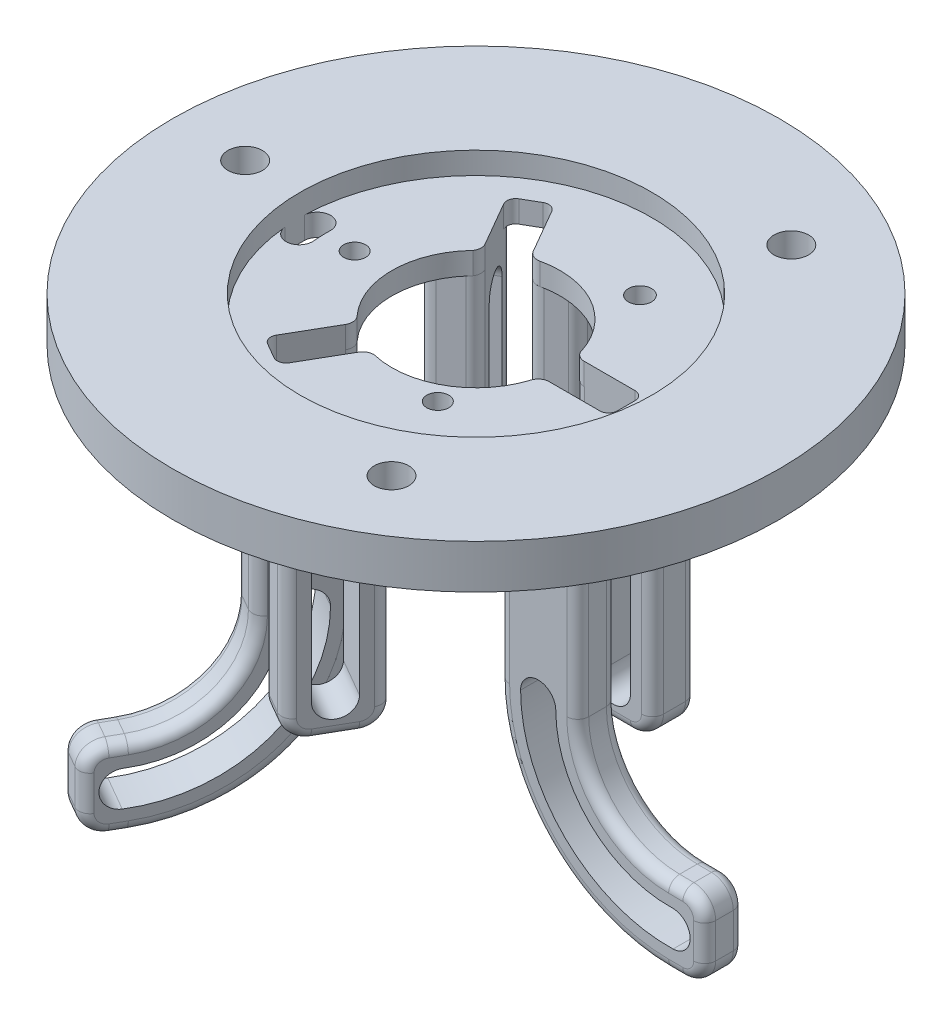
SolidWorks part; units mm, degrees
ref_plane "Front Plane" through (0, 0, 0) normal (0, 0, 1) x (1, 0, 0)
ref_plane "Top Plane" through (0, 0, 0) normal (0, 1, 0) x (1, 0, 0)
ref_plane "Right Plane" through (0, 0, 0) normal (1, 0, 0) x (0, 0, -1)
sketch "Sketch1" plane through (0, 0, 0) normal (0, 1, 0) x (1, 0, 0)
  circle A0 centre (0, 0) radius 138
extrude "Boss-Extrude1" add sketch "Sketch1" along normal blind 20
sketch "Sketch2" plane through (0, 0, 0) normal (0, 0, 1) x (1, 0, 0)
  line L0 (-138, 0) -> (138, 0) construction
  line L1 (62.2913, -161.1366) -> (62.2913, -17.2466)
  line L2 (54.2913, -100) -> (148.881, -100) construction
  line L3 (54.2913, -161.1366) -> (148.881, -161.1366) construction
  line L4 (113.6373, -189.6328) -> (113.6373, -71.1378) construction
  line L5 (113.6373, -71.1378) -> (113.6373, 30.2376) construction
  line L6 (138, 20) -> (138, 0) construction
  line L7 (54.2913, -161.1366) -> (54.2913, -17.2466) construction
  line L8 (46.2913, -161.1366) -> (46.2913, -17.2466)
  line L9 (36.2913, 0) -> (36.2913, -145.1821)
  line L10 (36.2913, -145.1821) -> (89.2746, -189.6328)
  line L11 (89.2746, -189.6328) -> (138, -189.6328)
  line L12 (82.2913, 0) -> (82.2913, -93.731)
  line L13 (82.2913, -93.731) -> (138, -149.4397)
  line L14 (138, -149.4397) -> (138, -189.6328)
  line L15 (138, 0) -> (138, -271.006) construction
  line L16 (36.2913, 0) -> (82.2913, 0)
  arc A0 (54.2913, -100) -> (113.6373, -159.346) centre (113.6373, -100) ccw construction
  arc A1 (54.2913, -161.1366) -> (113.6373, -220.4826) centre (113.6373, -161.1366) ccw construction
  arc A2 (62.2913, -161.1366) -> (113.6373, -212.4826) centre (113.6373, -161.1366) ccw
  arc A3 (46.2913, -100) -> (113.6373, -167.346) centre (113.6373, -100) ccw
  arc A4 (46.2913, -161.1366) -> (113.6373, -228.4826) centre (113.6373, -161.1366) ccw
  arc A5 (62.2913, -100) -> (113.6373, -151.346) centre (113.6373, -100) ccw
  arc A6 (113.6373, -212.4826) -> (113.6373, -228.4826) centre (113.6373, -220.4826) cw
  arc A7 (62.2913, -17.2466) -> (46.2913, -17.2466) centre (54.2913, -17.2466) ccw
  arc A8 (46.2913, -100) -> (62.2913, -100) centre (54.2913, -100) cw
  arc A9 (113.6373, -167.346) -> (113.6373, -151.346) centre (113.6373, -159.346) ccw
  circle A10 centre (54.2913, -161.1366) radius 8
  point P12 (113.6373, -100)
  point P14 (113.6373, -161.1366)
  point P15 (113.6373, -161.1366)
  dimension "D6" = 10
  dimension "D1" = 100
  dimension "D2" = 24.3627
  dimension "D3" = 61.1366
  dimension "D7" = 20
  dimension "D8" = 135
  dimension "D4" = 8
  dimension "D5" = 8
extrude "Boss-Extrude2" add sketch "Sketch2" along normal blind 10 and the other way blind 8 from offset 16 contours L16 L12 L13 L14 L11 L10 L9
sketch "Sketch3" plane through (0, 0, 26) normal (0, 0, 1) x (1, 0, 0)
  line L0 (54.2913, -17.2466) -> (54.2913, -110.5186) construction
  line L1 (46.2913, -17.2466) -> (46.2913, -110.5186)
  line L2 (62.2913, -17.2466) -> (62.2913, -110.5186)
  arc A0 (46.2913, -17.2466) -> (62.2913, -17.2466) centre (54.2913, -17.2466) cw
  arc A1 (46.2913, -110.5186) -> (62.2913, -110.5186) centre (54.2913, -110.5186) ccw
  dimension "D1" = 8
  dimension "D2" = 8
sketch "Sketch4" plane through (0, 0, 8) normal (0, 0, 1) x (1, 0, 0)
  arc A0 (54.2913, -100) -> (115.4184, -159.3192) centre (113.6373, -100) ccw
  arc A1 (54.2913, -100) -> (113.6373, -159.346) centre (113.6373, -100) ccw construction
  arc A2 (54.2913, -161.1366) -> (115.3389, -220.4582) centre (113.6373, -161.1366) ccw
  arc A3 (54.2913, -161.1366) -> (113.6373, -220.4826) centre (113.6373, -161.1366) ccw construction
  arc A4 (46.2913, -161.1366) -> (115.5682, -228.4549) centre (113.6373, -161.1366) ccw
  arc A5 (46.2913, -100) -> (115.6585, -167.3156) centre (113.6373, -100) ccw
  arc A6 (62.2913, -161.1366) -> (115.1095, -212.4615) centre (113.6373, -161.1366) ccw
  arc A7 (62.2913, -100) -> (115.1783, -151.3229) centre (113.6373, -100) ccw
  arc A8 (46.2913, -161.1366) -> (62.2913, -161.1366) centre (54.2913, -161.1366) cw
  arc A9 (115.5682, -228.4549) -> (115.1095, -212.4615) centre (115.3389, -220.4582) ccw
  arc A10 (46.2913, -100) -> (62.2913, -100) centre (54.2913, -100) cw
  arc A11 (115.6585, -167.3156) -> (115.1783, -151.3229) centre (115.4184, -159.3192) ccw
  dimension "D1" = 8
  dimension "D2" = 8
extrude "Cut-Extrude5" cut sketch "Sketch4" along normal blind 34
ref_plane "Plane1" through (0, 0, 42) normal (0, 0, 1) x (1, 0, 0)
sketch "Sketch7" plane through (0, 0, 42) normal (0, 0, 1) x (1, 0, 0)
  line L0 (36.2913, 0) -> (36.2913, -125.9674)
  line L1 (36.2913, 0) -> (36.2913, -145.1821) construction
  line L2 (36.2913, -125.9674) -> (82.2913, -125.9674)
  line L3 (82.2913, -125.9674) -> (82.2913, 0)
  line L4 (82.2913, 0) -> (36.2913, 0)
extrude "Boss-Extrude3" add sketch "Sketch7" along normal blind 20 from offset 70 contours L0 L2 L3 L4 offset against normal yes
extrude "Cut-Extrude6" cut sketch "Sketch3" along normal blind 45 from offset 72 offset against normal yes
sketch "Sketch8" plane through (0, 0, 26) normal (0, 0, 1) x (1, 0, 0)
  line L0 (130.0411, -141.4808) -> (130.0411, -169.783)
  line L1 (82.2913, -93.731) -> (138, -149.4397) construction
  line L2 (130.0411, -169.783) -> (130.0618, -195.2719)
  line L10 (130.065, -199.2899) -> (144.6927, -199.2899)
  line L11 (144.6927, -199.2899) -> (138, -149.4397)
  line L12 (138, -149.4397) -> (130.0411, -141.4808)
  line L13 (130.0618, -195.2719) -> (144.6927, -199.2899)
  line M11 (89.2746, -189.6328) -> (138, -189.6328)
  line M12 (138, -189.6328) -> (138, -149.4397)
  line M13 (138, -149.4397) -> (82.2913, -93.731)
extrude "Cut-Extrude7" cut sketch "Sketch8" against normal blind 72 contours L0 L2 M11 M12 M13
pattern_circular "CirPattern1" count 3 over 360 about axis through (0, 0, 0) along (0, 1, 0) of "Boss-Extrude3", "Cut-Extrude6", "Cut-Extrude5", "Boss-Extrude2", "Cut-Extrude7"
sketch "Sketch9" plane through (0, 0, -28) normal (0, 0, -1) x (-1, 0, 0)
  line L4 (-72.2913, -43.2737) -> (-72.2913, 0)
  line L5 (-82.2913, 0) -> (-36.2913, 0) construction
  line L6 (-72.2913, -43.2737) -> (-72.2913, -125.9674)
  line L7 (-36.2913, -125.9674) -> (-82.2913, -125.9674) construction
  line L8 (-72.2913, -125.9674) -> (-82.2913, -125.9674)
  line L9 (-82.2913, -125.9674) -> (-82.2913, 0)
  line L10 (-82.2913, 0) -> (-72.2913, 0)
extrude "Cut-Extrude8" cut sketch "Sketch9" against normal blind 27
sketch "Sketch11" plane through (0, 0, 26) normal (0, 0, 1) x (1, 0, 0)
  line L0 (36.2913, -100) -> (36.2913, -145.1821)
  line L1 (36.2913, -145.1821) -> (89.2746, -189.6328)
  line L2 (89.2746, -189.6328) -> (130.0572, -189.6328)
  line L3 (130.0572, -189.6328) -> (134.4943, -177.346)
  line L5 (72.2873, -100) -> (72.2873, 0)
  line L6 (36.2913, 0) -> (82.2913, 0) construction
  line L7 (72.2873, 0) -> (138, 0)
  line L8 (138, 0) -> (154.9873, -100)
  line L9 (113.6373, -141.35) -> (130.0411, -141.4808)
  line L10 (130.0411, -141.4808) -> (142.1558, -129.9419)
  line L11 (113.6373, -177.346) -> (134.4943, -177.346)
  arc A0 (36.2913, -100) -> (113.6373, -177.346) centre (113.6373, -100) ccw
  arc A1 (72.2873, -100) -> (113.6373, -141.35) centre (113.6373, -100) ccw
  arc A2 (142.1558, -129.9419) -> (154.9873, -100) centre (113.6373, -100) ccw
  dimension "D1" = 82.7
extrude "Cut-Extrude10" cut sketch "Sketch11" against normal blind 27
pattern_circular "CirPattern4" count 3 over 360 about axis through (0, 20, 0) along (0, -1, 0) of "Cut-Extrude8"
pattern_circular "CirPattern5" count 3 over 360 about axis through (0, 0, 0) along (0, 1, 0) of "Cut-Extrude10"
fillet "Fillet2" radius 10 21 edges at (-2.5572, -125.9674, 40.4292) (-33.7341, -125.9674, -22.4292) (-79.743, -169.783, 104.1189) (-79.743, -141.4808, 104.1189) (-71.9503, -173.5645, 108.6215) (-87.5387, -173.5645, 99.6215) (-50.2981, -169.783, -121.1189) (-50.2981, -141.4808, -121.1189) (-58.0939, -173.5645, -116.6215) (-42.5054, -173.5645, -125.6215) (72.2913, -125.9674, -18) (130.0472, -177.346, 17) (-51.7341, -125.9674, -53.6061) (-20.5572, -125.9674, 71.6061) (-79.746, -177.346, 104.1242) (-50.3012, -177.346, -121.1242) (36.2913, -125.9674, -18) (130.0411, -169.783, 17) (130.0411, -141.4808, 17) (130.0441, -173.5645, 8) (130.0441, -173.5645, 26)
sketch "Sketch12" plane through (0, 20, 0) normal (0, 1, 0) x (1, 0, 0)
  line L0 (0, 0) -> (-105, 0) construction
  line L1 (0, 0) -> (0, 105) construction
  circle A0 centre (0, 0) radius 105 construction
  circle A2 centre (-105, 0) radius 7.875
  dimension "D1" = 210
  dimension "D2" = 15.75
  dimension "D3" = 90
extrude "Cut-Extrude11" cut sketch "Sketch12" against normal blind 27
pattern_circular "CirPattern8" count 3 over 360 about axis through (0, 0, 0) along (0, 1, 0) of "Cut-Extrude11"
fillet "Fillet3" radius 5 84 edges at (-25.0739, -50, 27.4292) (36.2913, -50, 26) (-40.6623, -50, 18.4292) (-11.2175, -50, -35.4292) (4.371, -50, -44.4292) (6.103, -57.9837, 45.4292) (-11.2175, -57.9837, 35.4292) (-42.3944, -57.9837, -17.4292) (-25.0739, -57.9837, -27.4292) (72.2913, -57.9837, -8) (58.9454, -154.6919, 8) (58.9454, -154.6919, 26) (72.2873, -50, 26) (84.3984, -129.2389, 26) (116.879, -141.3758, 26) (84.3984, -129.2389, 8) (72.2873, -50, 8) (116.879, -141.3758, 8) (-43.0739, -57.9837, -58.6061) (-29.2175, -57.9837, 66.6061) (-22.5445, -154.6919, -55.0482) (-6.9561, -154.6919, -64.0482) (-58.6603, -50, 49.6026) (-64.7159, -129.2389, 60.0912) (-80.9562, -141.3758, 88.2202) (-49.1274, -129.2389, 69.0912) (-43.0719, -50, 58.6026) (-65.3677, -141.3758, 97.2202) (-36.4009, -154.6919, 47.0482) (-51.9894, -154.6919, 38.0482) (36.2913, -57.9837, -28) (-13.627, -50, -75.6026) (-19.6826, -129.2389, -86.0912) (-35.9229, -141.3758, -114.2202) (-35.271, -129.2389, -77.0912) (-29.2155, -50, -66.6026) (-51.5113, -141.3758, -105.2202) (36.2913, -57.9837, -8) (-42.5039, -159.3737, -125.6189) (-58.0923, -159.3737, -116.6189) (-35.9029, -177.346, -114.1857) (-41.0394, -174.4171, -123.0823) (-41.0535, -144.3585, -123.1067) (-51.4914, -177.346, -105.1857) (-56.6279, -174.4171, -114.0823) (-56.6419, -144.3585, -114.1067) (-87.5372, -159.3737, 99.6189) (-71.9487, -159.3737, 108.6189) (-80.9363, -177.346, 88.1857) (-86.0727, -174.4171, 97.0823) (-86.0868, -144.3585, 97.1067) (-65.3478, -177.346, 97.1857) (-70.4843, -174.4171, 106.0823) (-70.4983, -144.3585, 106.1067) (-60.3944, -57.9837, -48.6061) (-51.3944, -125.9674, -33.0177) (-43.8588, -123.0385, -19.9657) (-58.9299, -123.0385, -46.0696) (-34.0739, -125.9674, -43.0177) (-26.5383, -123.0385, -29.9657) (-41.6094, -123.0385, -56.0696) (-2.897, -125.9674, 61.0177) (-20.2175, -125.9674, 51.0177) (-11.897, -57.9837, 76.6061) (-10.4325, -123.0385, 74.0696) (4.6386, -123.0385, 47.9657) (-27.753, -123.0385, 64.0696) (-12.6819, -123.0385, 37.9657) (54.2913, -125.9674, -28) (54.2913, -125.9674, -8) (72.2913, -57.9837, -28) (69.3624, -123.0385, -28) (39.2203, -123.0385, -28) (69.3624, -123.0385, -8) (39.2203, -123.0385, -8) (130.0411, -159.3737, 26) (130.0411, -159.3737, 8) (116.8392, -177.346, 26) (127.1121, -174.4171, 26) (127.1403, -144.3585, 26) (116.8392, -177.346, 8) (127.1121, -174.4171, 8) (127.1403, -144.3585, 8) (36.2913, -50, 8)
sketch "Sketch13" plane through (0, 0, 0) normal (0, -1, 0) x (1, 0, 0)
  line L0 (-39.0867, 51.7001) -> (-25.6504, 28.4278)
  line L2 (-27.5739, 31.7593) -> (-40.5719, 54.2725) construction
  line L4 (-25.2303, 59.7001) -> (-11.794, 36.4278)
  line L6 (-37.6226, 57.1642) -> (-30.6944, 61.1642)
  line L7 (64.3169, -8) -> (37.4444, -8)
  line L8 (68.3169, 4) -> (68.3169, -4)
  line L9 (64.3169, 8) -> (37.4444, 8)
  line L10 (-39.0867, -51.7001) -> (-25.6504, -28.4278)
  line L11 (-30.6944, -61.1642) -> (-37.6226, -57.1642)
  line L12 (-25.2303, -59.7001) -> (-11.794, -36.4278)
  arc A0 (-25.6504, 28.4278) -> (-25.6504, -28.4278) centre (0, 0) ccw
  arc A1 (37.4444, 8) -> (-11.794, 36.4278) centre (0, 0) ccw
  arc A2 (-11.794, -36.4278) -> (37.4444, -8) centre (0, 0) ccw
  arc A3 (-25.2303, 59.7001) -> (-30.6944, 61.1642) centre (-28.6944, 57.7001) ccw
  arc A4 (68.3169, 4) -> (64.3169, 8) centre (64.3169, 4) ccw
  arc A5 (68.3169, -4) -> (64.3169, -8) centre (64.3169, -4) cw
  arc A6 (-37.6226, -57.1642) -> (-39.0867, -51.7001) centre (-35.6226, -53.7001) cw
  arc A7 (-39.0867, 51.7001) -> (-37.6226, 57.1642) centre (-35.6226, 53.7001) cw
  arc A8 (-30.6944, -61.1642) -> (-25.2303, -59.7001) centre (-28.6944, -57.7001) ccw
  point P18 (0, 0)
  dimension "D2" = 4
  dimension "D3" = 4
  dimension "D4" = 4
  dimension "D1" = 3
extrude "Cut-Extrude12" cut sketch "Sketch13" against normal blind 27
sketch "Sketch14" plane through (0, 0, 0) normal (0, -1, 0) x (1, 0, 0)
  line L0 (-27.5739, 31.7593) -> (-13.7175, 39.7593)
  line L3 (41.2913, 8) -> (41.2913, -8)
  line L4 (-13.7175, -39.7593) -> (-27.5739, -31.7593)
  arc A0 (-13.7175, 39.7593) -> (-8.9941, 37.2181) centre (-9.3271, 42.2593) ccw
  arc A1 (-27.5739, 31.7593) -> (-28.1914, 25.9099) centre (-31.9042, 29.2592) cw
  arc A2 (-28.219, 25.8798) -> (-28.219, -25.8798) centre (0, 0) ccw construction
  arc A3 (-25.6504, 28.4278) -> (-28.219, 25.8798) centre (0, 0) ccw construction
  arc A4 (-28.1914, 25.9099) -> (-27.7347, -26.3982) centre (0, 0) ccw
  arc A6 (41.2913, 8) -> (36.5344, 11.4595) centre (41.2913, 13.0003) cw
  arc A7 (41.2913, -8) -> (36.7289, -10.8199) centre (41.2612, -13.0522) ccw
  arc A8 (-13.7175, -39.7593) -> (-8.343, -37.3694) centre (-9.3871, -42.2595) cw
  arc A9 (-27.5739, -31.7593) -> (-27.7347, -26.3982) centre (-31.9341, -29.2072) ccw
  arc A10 (36.5344, 11.4595) -> (-8.9941, 37.2181) centre (0, 0) ccw
  arc A11 (-8.343, -37.3694) -> (36.7289, -10.8199) centre (0, 0) ccw
  point P31 (0, 0)
  dimension "D1" = 3
extrude "Cut-Extrude13" cut sketch "Sketch14" against normal blind 27
sketch "Sketch17" plane through (0, 20, 0) normal (0, 1, 0) x (1, 0, 0)
  circle A0 centre (0, 0) radius 80
  dimension "D1" = 160
extrude "Cut-Extrude14" cut sketch "Sketch17" against normal blind 10
sketch "Sketch18" plane through (0, 10, 0) normal (0, 1, 0) x (1, 0, 0)
  arc A0 (-73.6973, -6.6862) -> (-73.9778, 1.812) centre (0, 0) cw construction
  arc A1 (-79.976, 1.959) -> (-79.6728, -7.2283) centre (0, 0) ccw
  arc A2 (-67.9796, 1.6651) -> (-67.7219, -6.144) centre (0, 0) ccw
  arc A3 (-67.9796, 1.6651) -> (-79.976, 1.959) centre (-73.9778, 1.812) ccw
  arc A4 (-79.6728, -7.2283) -> (-67.7219, -6.144) centre (-73.6973, -6.6862) ccw
  circle A5 centre (0, 0) radius 80 construction
  point P4 (-73.9597, -2.4411)
  dimension "D1" = 68
extrude "Cut-Extrude15" cut sketch "Sketch18" against normal blind 10
sketch "Sketch19" plane through (0, 10, 0) normal (0, 1, 0) x (1, 0, 0)
  circle A0 centre (23.75, -41.1362) radius 5
  circle A1 centre (27.8862, 46.6997) radius 5.2694
  circle A2 centre (-54.3862, -0.8003) radius 5
extrude "Cut-Extrude16" cut sketch "Sketch19" against normal blind 10
